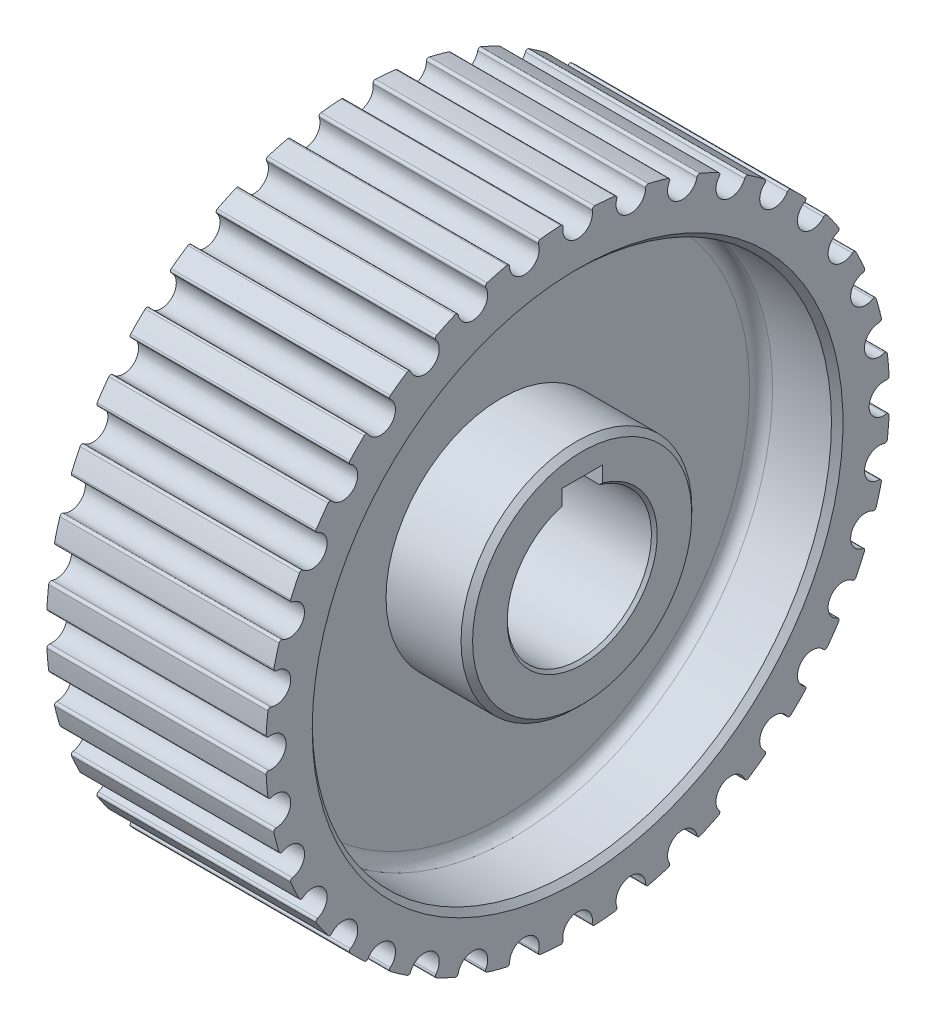
from build123d import *

# Parameters (mm, degrees)
CHAMFER_1_SIZE           = 1
FILLET_1_R               = 2
CHAMFER_2_SIZE           = 1
CHAMFER_3_SIZE           = 0.5
CUT_EXTRUDE_1_DEPTH      = 86.744329753
CUT_EXTRUDE_2_DEPTH      = 86.744329753
PATTERN_CIRCULAR_2_COUNT = 36


with BuildPart() as part:
    # 草图1 → 旋转1 (revolve)
    with BuildSketch(Plane.XY, mode=Mode.PRIVATE) as revolve_1_sk:
        Polygon((-20.32928411, 12.5), (17.67071589, 12.5), (17.67071589, 20), (3.67071589, 20), (3.67071589, 45), (16.876898279, 45), (16.876898279, 54.07), (-21.123101721, 54.07), (-21.123101721, 45), (-6.32928411, 45), (-6.32928411, 20), (-20.32928411, 20), align=None)
    revolve(revolve_1_sk.sketch.rotate(Axis((-38.472219195, 0, 0), (1, 0, 0)), 90), axis=Axis((-38.472219195, 0, 0), (1, 0, 0)))

    # 倒角1
    chamfer_1_edges = [part.edges().sort_by_distance(p)[0] for p in [
        (16.876898279, 0, -45),
        (-21.123101721, 0, -45),
    ]]
    chamfer(chamfer_1_edges, length=CHAMFER_1_SIZE)

    # 圆角1
    fillet_1_edges = [part.edges().sort_by_distance(p)[0] for p in [
        (3.67071589, 0, -45),
        (-6.32928411, 0, -45),
    ]]
    fillet(fillet_1_edges, radius=FILLET_1_R)

    # 倒角2
    chamfer_2_edges = [part.edges().sort_by_distance(p)[0] for p in [
        (17.67071589, 0, -20),
        (-20.32928411, 0, -20),
    ]]
    chamfer(chamfer_2_edges, length=CHAMFER_2_SIZE)

    # 倒角3
    chamfer_3_edges = [part.edges().sort_by_distance(p)[0] for p in [
        (17.67071589, 0, -12.5),
        (-20.32928411, 0, -12.5),
    ]]
    chamfer(chamfer_3_edges, length=CHAMFER_3_SIZE)

    # 草图2 → 切除-拉伸1 (cut, through all)
    with BuildSketch(Plane(origin=(17.67071589, 0, 0), x_dir=(0, 0, -1), z_dir=(1, 0, 0))):
        with BuildLine():
            Line((-3.5, 12), (-3.5, 15.2))
            Line((-3.5, 15.2), (3.5, 15.2))
            Line((3.5, 15.2), (3.5, 12))
            ThreePointArc((3.5, 12), (0, 12.5), (-3.5, 12))
        make_face()
    extrude(amount=-CUT_EXTRUDE_1_DEPTH, mode=Mode.SUBTRACT)

    # 草图5 → 切除-拉伸2 (cut, symmetric)
    with BuildSketch(Plane.ZY.offset(21.123101721)):
        with BuildLine():
            ThreePointArc((-2.534781705, 53.524006734), (0, 50.53), (2.534781705, 53.524006734))
            ThreePointArc((2.534781705, 53.524006734), (2.631185469, 53.856697531), (2.951132196, 53.989403764))
            ThreePointArc((2.951132196, 53.989403764), (0, 54.07), (-2.951132196, 53.989403764))
            ThreePointArc((-2.951132196, 53.989403764), (-2.631185469, 53.856697531), (-2.534781705, 53.524006734))
        make_face()
    cut_extrude_2 = extrude(amount=CUT_EXTRUDE_2_DEPTH, both=True, mode=Mode.SUBTRACT)

    # 阵列(圆周)2: 切除-拉伸2 ×36 about axis
    pattern_circular_2_axis = Axis((0, 0, 0), (1, 0, 0))
    for i in range(1, PATTERN_CIRCULAR_2_COUNT):
        add(cut_extrude_2.rotate(pattern_circular_2_axis, i * 360 / PATTERN_CIRCULAR_2_COUNT), mode=Mode.SUBTRACT)


solid = part.part
